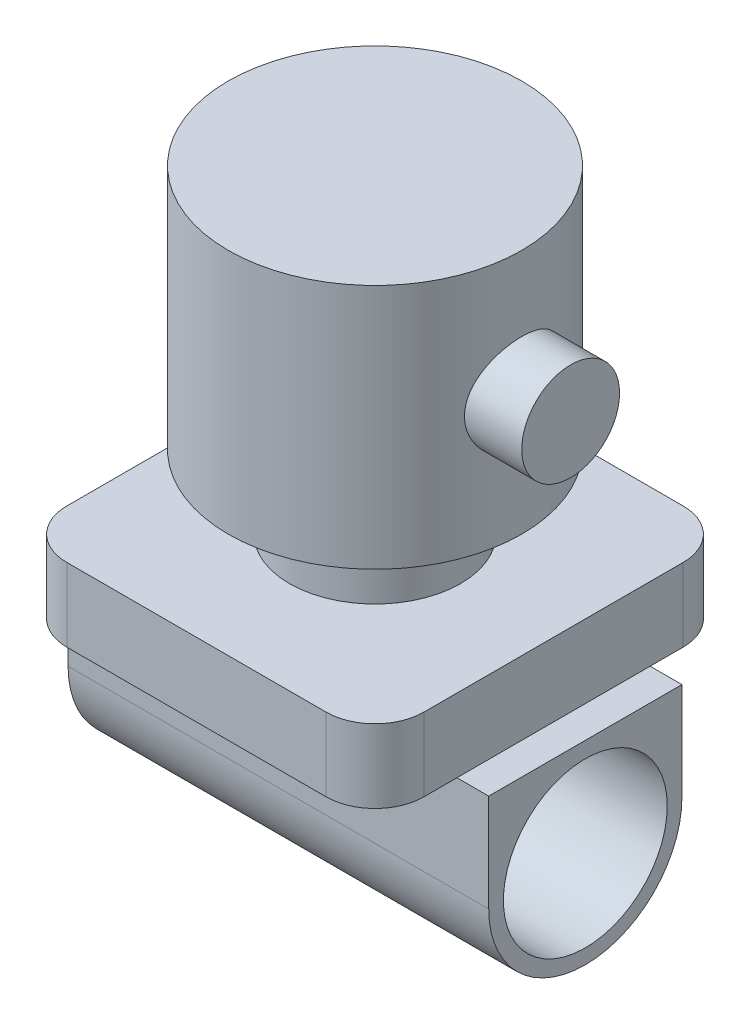
from build123d import *

# Parameters (mm, degrees)
SKETCH_1_R           = 19.75
SKETCH_1_R_2         = 16.75
EXTRUDE_1_DEPTH      = 43
EXTRUDE_1_2_DEPTH    = 15
SKETCH_4_R           = 17.5
EXTRUDE_2_DEPTH      = 15
SKETCH_5_R           = 30
EXTRUDE_3_DEPTH      = 50.25
EXTRUDE_START        = -86
EXTRUDE_4_DEPTH      = 86
EXTRUDE_5_REACH      = 137.171
EXTRUDE_5_END_RADIUS = 30
SKETCH_7_R           = 10


with BuildPart() as part:
    # 草图1 → Extrude 1 (new, symmetric)
    with BuildSketch(Plane(origin=(0, 0, 0), x_dir=(0, 0, -1), z_dir=(1, 0, 0))):
        Circle(SKETCH_1_R)
        Circle(SKETCH_1_R_2, mode=Mode.SUBTRACT)
    extrude(amount=EXTRUDE_1_DEPTH, both=True)



with BuildPart() as body_2:
    # 草图3 → Extrude 1 2 (new body)
    with BuildSketch(Plane(origin=(0, 20, 0), x_dir=(1, 0, 0), z_dir=(0, 1, 0))):
        with BuildLine():
            Line((-26.5, 36.5), (26.5, 36.5))
            ThreePointArc((26.5, 36.5), (33.571067812, 33.571067812), (36.5, 26.5))
            Line((36.5, 26.5), (36.5, -26.5))
            ThreePointArc((36.5, -26.5), (33.571067812, -33.571067812), (26.5, -36.5))
            Line((26.5, -36.5), (-26.5, -36.5))
            ThreePointArc((-26.5, -36.5), (-33.571067812, -33.571067812), (-36.5, -26.5))
            Line((-36.5, -26.5), (-36.5, 26.5))
            ThreePointArc((-36.5, 26.5), (-33.571067812, 33.571067812), (-26.5, 36.5))
        make_face()
    extrude(amount=EXTRUDE_1_2_DEPTH)

    # 草图4 → 凸台-拉伸2 (add)
    with BuildSketch(Plane(origin=(0, 35, 0), x_dir=(1, 0, 0), z_dir=(0, 1, 0))):
        with Locations(Location((0, 0, 0), (0, 0, 90))):
            Circle(SKETCH_4_R)
    extrude(amount=EXTRUDE_2_DEPTH)

    # 草图5 → 凸台-拉伸3 (add)
    with BuildSketch(Plane(origin=(0, 50, 0), x_dir=(1, 0, 0), z_dir=(0, 1, 0))):
        with Locations(Location((0, 0, 0), (0, 0, 270))):
            Circle(SKETCH_5_R)
    extrude(amount=EXTRUDE_3_DEPTH)


with BuildPart() as part_1:
    add(part.part)

    add(body_2.part)  # 凸台-拉伸4 merges body 2
    # 草图6 → 凸台-拉伸4 (add)
    with BuildSketch(Plane(origin=(43, 0, 0), x_dir=(0, 0, -1), z_dir=(1, 0, 0)).offset(EXTRUDE_START)):
        with BuildLine():
            Line((-19.75, 0), (-19.75, 20))
            Line((-19.75, 20), (19.75, 20))
            Line((19.75, 20), (19.75, 0))
            ThreePointArc((19.75, 0), (0, 19.75), (-19.75, 0))
        make_face()
    extrude(amount=EXTRUDE_4_DEPTH)

    # 凸台-拉伸5: up to this cylinder (the profile starts outside it)
    extrude_5_end = Plane(origin=(0, 75, 0), z_dir=(0, -1, 0)) * Cylinder(EXTRUDE_5_END_RADIUS, 335.342, mode=Mode.PRIVATE)
    # 草图7 → 凸台-拉伸5 (add, up to the surface)
    with BuildSketch(Plane(origin=(40, 0, 0), x_dir=(0, 0, -1), z_dir=(1, 0, 0)), mode=Mode.PRIVATE) as extrude_5_sk1:
        with Locations((0, 75)):
            Circle(SKETCH_7_R)
    extrude_5_tool1 = extrude(extrude_5_sk1.sketch, amount=-EXTRUDE_5_REACH, mode=Mode.PRIVATE) - extrude_5_end
    add(extrude_5_tool1.solids().sort_by_distance((40, 75, 0))[0])


solid = part_1.part
